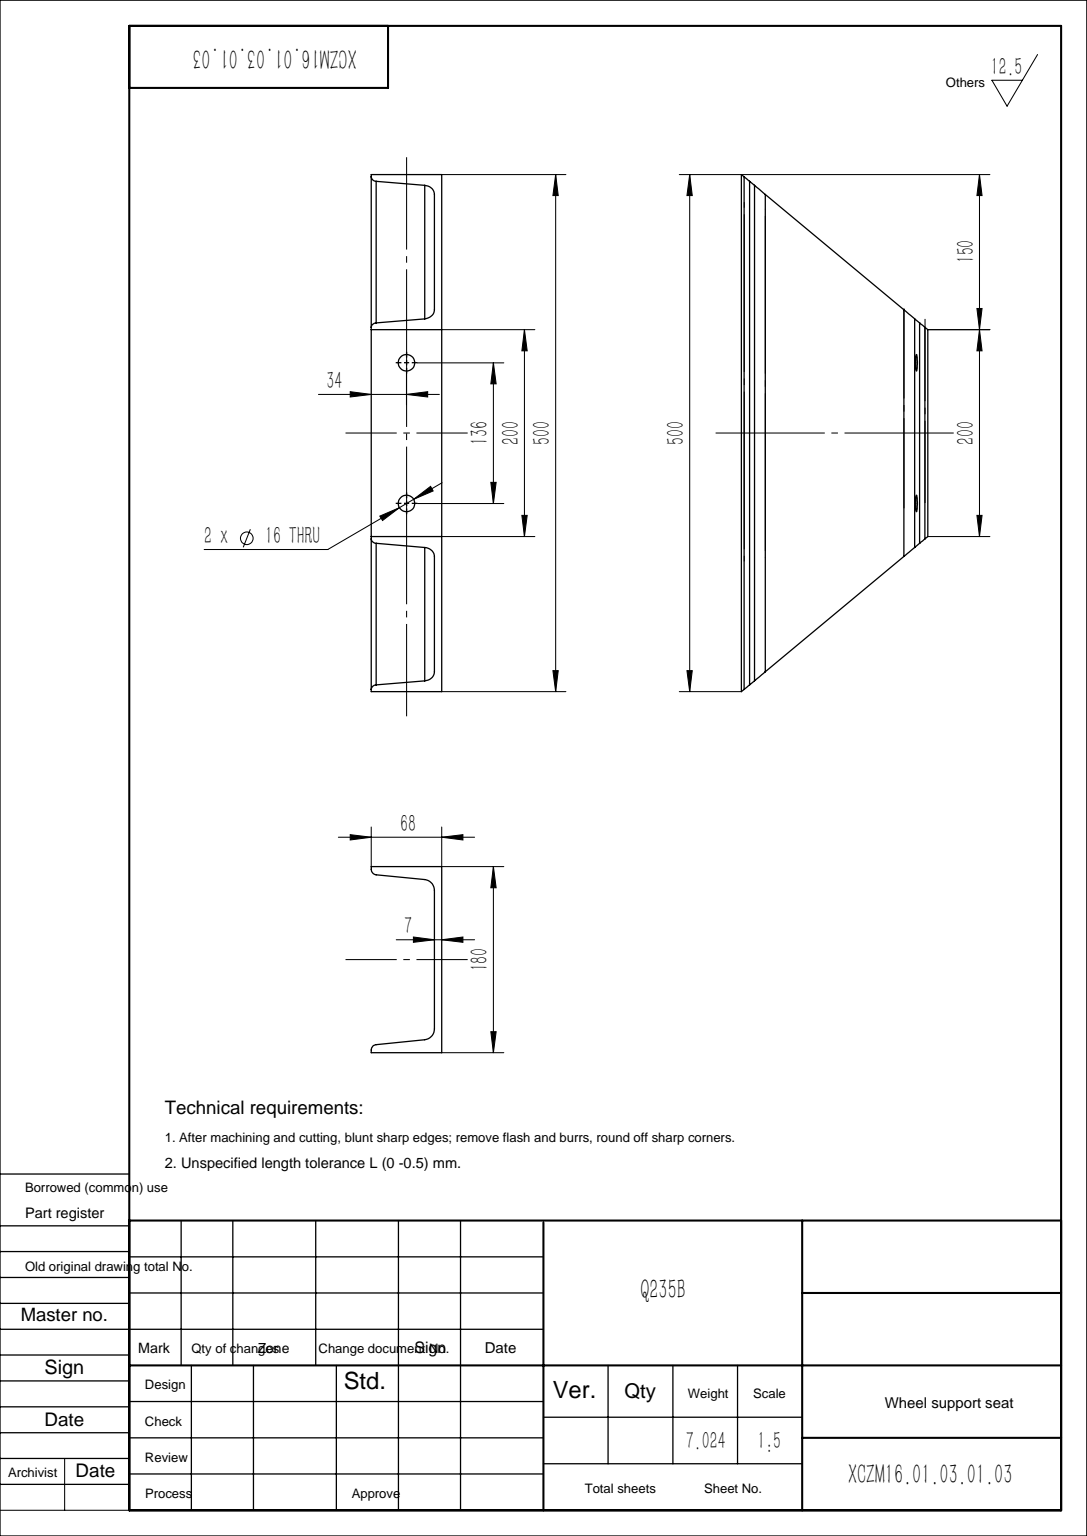
SolidWorks part; units mm, degrees
material "XRAAT"
ref_plane "前视基准面" through (0, 0, 0) normal (0, 0, 1) x (1, 0, 0)
ref_plane "上视基准面" through (0, 0, 0) normal (0, 1, 0) x (1, 0, 0)
ref_plane "右视基准面" through (0, 0, 0) normal (1, 0, 0) x (0, 0, -1)
sketch "草图1" plane through (0, 0, 0) normal (0, 0, 1) x (1, 0, 0)
  line L0 (0, 0) -> (0, 500)
  dimension "D1" = 500
other "热轧普通槽钢(gb t707-1988) 18A-XXXXXXXXXXXXXXX528V9(2)"
ref_plane "基准面1" through (0, 0, 0) normal (0, 1, 0) x (-1, 0, 0)
sketch "Sketch11" plane through (0, 0, 0) normal (0, 1, 0) x (-1, 0, 0)
  line L0 (68, 180) -> (0, 180)
  line L1 (68, 0) -> (0, 0)
  line L2 (0, 180) -> (0, 0)
  line L3 (54.084, 120.3761) -> (64.084, 120.3761) construction
  line L4 (54.084, 120.3761) -> (54.084, 119.3761) construction
  line L5 (54.084, 119.3761) -> (64.084, 120.3761) construction
  line L6 (68, 180) -> (68, 177.3012)
  line L7 (68, 0) -> (68, 2.6988)
  line L8 (0, 90) -> (7, 90) construction
  line L9 (37.5, 169.5) -> (37.5, 180) construction
  line L10 (7, 156.9476) -> (7, 169.5) construction
  line L11 (7, 169.5) -> (68, 169.5) construction
  line L12 (7, 156.9476) -> (7, 23.0524)
  line L13 (68, 169.5) -> (68, 180) construction
  line L17 (16.4552, 167.3955) -> (63.2724, 172.0772)
  line L18 (16.4552, 12.6045) -> (63.2724, 7.9228)
  arc A0 (63.2724, 172.0772) -> (68, 177.3012) centre (62.75, 177.3012) ccw
  arc A1 (63.2724, 7.9228) -> (68, 2.6988) centre (62.75, 2.6988) cw
  arc A9 (7, 23.0524) -> (16.4552, 12.6045) centre (17.5, 23.0524) ccw
  arc A10 (7, 156.9476) -> (16.4552, 167.3955) centre (17.5, 156.9476) cw
  point P8 (0, 90)
  point P9 (7, 90)
  point P10 (34, 180)
  point P11 (34, 0)
  point P12 (68, 7.45)
  point P13 (68, 172.55)
  point P27 (0, 0)
  dimension "D4" = 68
  dimension "D5" = 7
  dimension "D2" = 10
  dimension "D8" = 10.5
  dimension "D3" = 180
  dimension "D6" = 10.5
  dimension "D7" = 5.25
  dimension "D1" = 1
sketch "草图8" plane through (0, 0, 180) normal (-1, 0, 0) x (0, 0, 1)
  line L0 (0, 500) -> (-180, 350)
  line L1 (-180, 0) -> (-180, 500) construction
  line L2 (-180, 350) -> (-180, 500)
  line L3 (-180, 500) -> (0, 500)
  line L4 (-180, 250) -> (0, 250) construction
  line L5 (0, 500) -> (0, 0) construction
  line L6 (-180, 0) -> (0, 0)
  line L7 (-180, 150) -> (-180, 0)
  line L8 (0, 0) -> (-180, 150)
  dimension "D1" = 200
extrude "切除-拉伸1" cut sketch "草图8" along normal through all
hole_wizard "Ø16.0 (16) 直径孔1" positions "草图9" profile "草图10" hole size "Ø16.0" standard "GB"
sketch "草图9" plane through (0, 0, 0) normal (0, 0, -1) x (-1, 0, 0)
  line L0 (0, 250) -> (16.4552, 250) construction
  line L1 (0, 0) -> (0, 500) construction
  line L2 (16.4552, 360.5037) -> (16.4552, 139.4963) construction
  point P0 (34, 318)
  point P10 (34, 182)
  dimension "D1" = 34
  dimension "D2" = 136
sketch "草图10" plane through (-34, 318, 0) normal (1, 0, 0) x (0, 1, 0)
  line L0 (0, 0) -> (0, 10.85)
  line L1 (0, 10.85) -> (8, 10.85)
  line L2 (8, 10.85) -> (8, 0)
  line L5 (8, 0) -> (0, 0)
  line L11 (0, -6.35) -> (0, 107.95) construction
  dimension "通孔孔直径" = 16
  dimension "通孔孔深度" = 10.85
